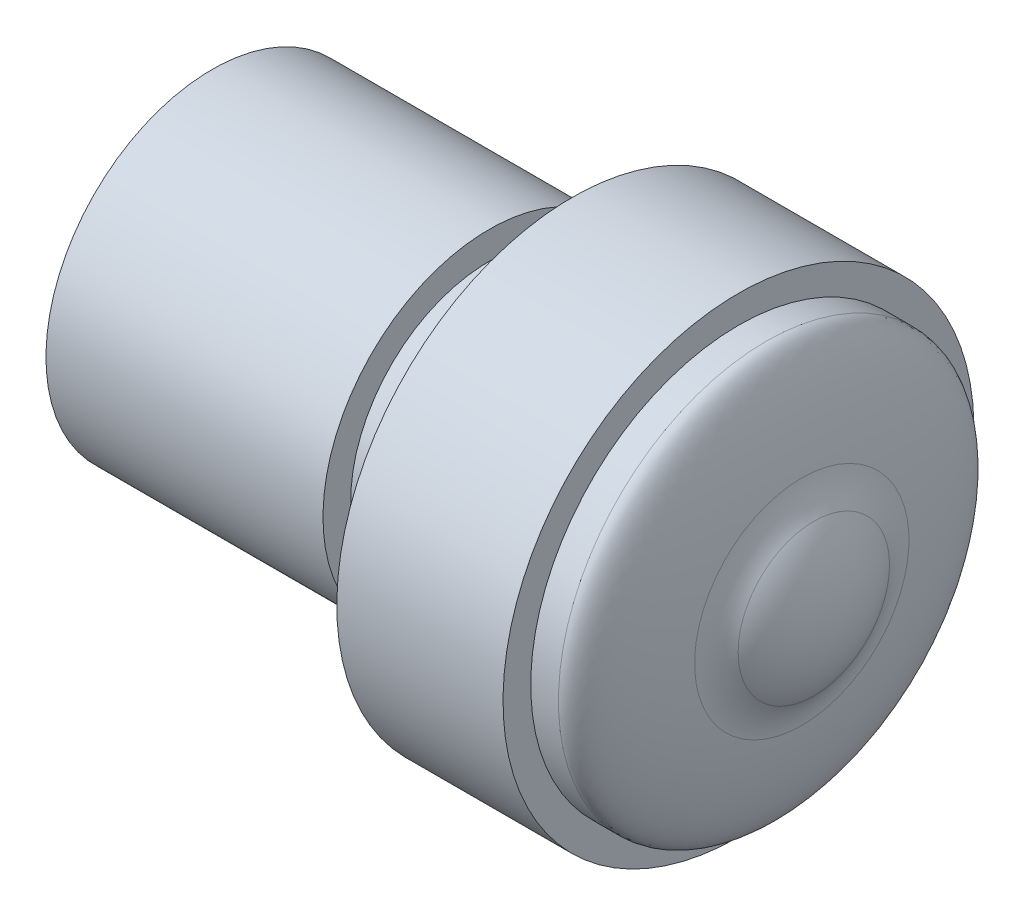
from build123d import *


with BuildPart() as part:
    # Sketch1 → Revolve1 (revolve)
    with BuildSketch(Plane.XY, mode=Mode.PRIVATE) as revolve1_sk:
        with BuildLine():
            Line((0, 0), (0, 12))
            Line((0, 12), (20, 12))
            Line((20, 12), (20, 10))
            Line((20, 10), (25.99851273, 10))
            Line((25.99851273, 10), (25.99851273, 17))
            Line((25.99851273, 17), (37.99851273, 17))
            Line((37.99851273, 17), (37.99851273, 15))
            Line((37.99851273, 15), (39.99851273, 15))
            add(Edge.make_bspline(
                [(42.56851273, 7.738055311), (41.693908377, 15), (39.99851273, 15)],
                knots=[2.112819643, 2.112819643, 2.112819643, 3.141592654, 3.141592654, 3.141592654], degree=2, weights=[1, 0.870594726, 1]))
            ThreePointArc((42.56851273, 7.738055311), (42.863176718, 6.548150813), (43.43851273, 5.465705407))
            add(Edge.make_bspline(
                [(45, 0), (45, 3.238369631), (43.43851273, 5.465705407)],
                knots=[4.71238898, 4.71238898, 4.71238898, 5.524737662, 5.524737662, 5.524737662], degree=2, weights=[1, 0.918639051, 1]))
            Line((45, 0), (0, 0))
        make_face()
    revolve(revolve1_sk.sketch.rotate(Axis((0, 0, 0), (1, 0, 0)), 180), axis=Axis((0, 0, 0), (1, 0, 0)))


solid = part.part
